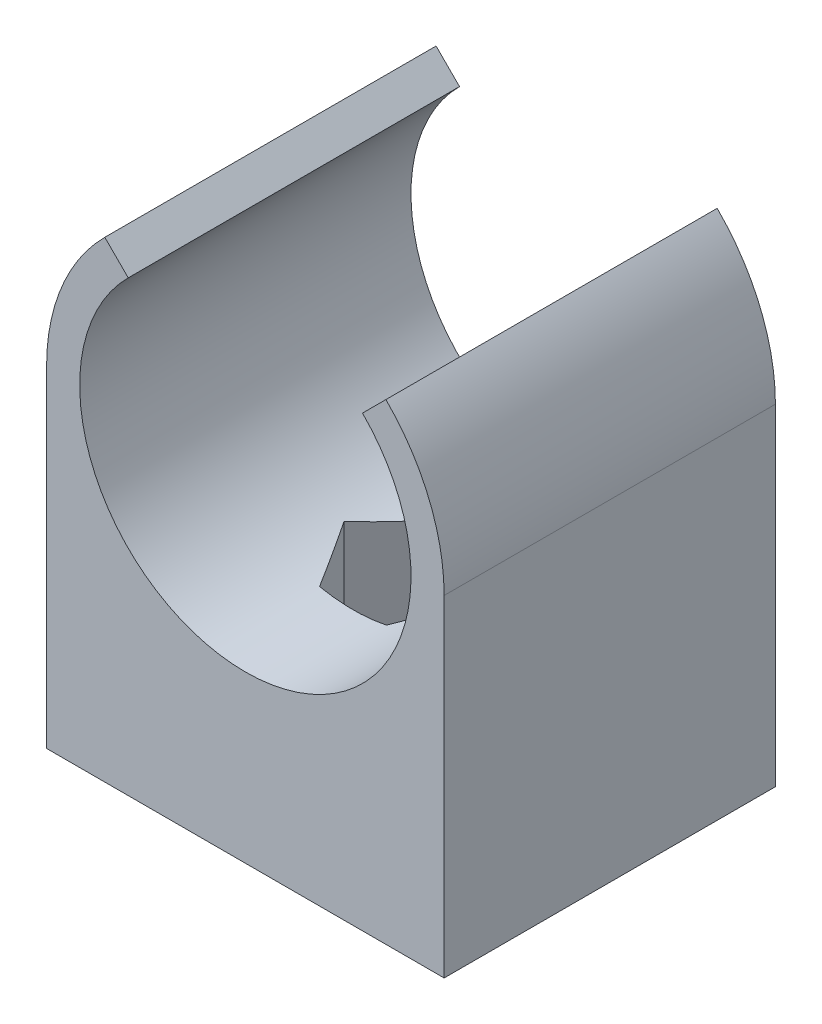
SolidWorks part; units mm, degrees
material "PP 共聚物"
ref_plane "前视基准面" through (0, 0, 0) normal (0, 0, 1) x (1, 0, 0)
ref_plane "上视基准面" through (0, 0, 0) normal (0, 1, 0) x (1, 0, 0)
ref_plane "右视基准面" through (0, 0, 0) normal (1, 0, 0) x (0, 0, -1)
sketch "草图1" plane through (0, 0, 0) normal (0, 0, 1) x (1, 0, 0)
  line L0 (-12, 10) -> (-12, 20)
  line L2 (-12, 10) -> (-12, 0)
  line L3 (-12, 0) -> (12, 0)
  line L4 (12, 10) -> (12, 0)
  line L5 (-7.0711, 27.0711) -> (-8.4853, 28.4853)
  line L6 (0, 41.9292) -> (0, 30) construction
  line L7 (12, 10) -> (12, 20)
  line L8 (7.0711, 27.0711) -> (8.4853, 28.4853)
  line L11 (0, 20) -> (0, -7.785) construction
  arc A0 (-7.0711, 27.0711) -> (7.0711, 27.0711) centre (0, 20) ccw
  arc A1 (-8.4853, 28.4853) -> (-12, 20) centre (0, 20) ccw
  arc A2 (12, 20) -> (8.4853, 28.4853) centre (0, 20) ccw
  dimension "D4" = 20
  dimension "D1" = 10
  dimension "D2" = 24
  dimension "D3" = 12
  dimension "D5" = 45
  dimension "D6" = 45
extrude "凸台-拉伸1" add sketch "草图1" along normal blind 20
hole_wizard "Ø5.0 (5) 直径孔1" positions "草图5" profile "草图6" hole size "Ø5.0" standard "Gb" end condition through all
sketch "草图5" plane through (0, 0, 0) normal (0, -1, 0) x (-1, 0, 0)
  line L0 (-12, -20) -> (-12, 0) construction
  line L2 (12, -20) -> (-12, -20) construction
  point P0 (0, -10)
  dimension "D1" = 12
  dimension "D2" = 10
sketch "草图6" plane through (0, 0, 10) normal (1, 0, 0) x (0, 0, -1)
  line L0 (0, 0) -> (0, 28.4853)
  line L1 (0, 28.4853) -> (2.5, 28.4853)
  line L2 (2.5, 28.4853) -> (2.5, 0)
  line L5 (2.5, 0) -> (0, 0)
  line L11 (0, -6.35) -> (0, 107.95) construction
  dimension "通孔孔直径" = 5
  dimension "通孔孔深度" = 28.4853
ref_plane "基准面1" through (0, 10, 0) normal (0, -1, 0) x (-1, 0, 0)
sketch "草图7" plane through (0, 10, 0) normal (0, -1, 0) x (-1, 0, 0)
  line L1 (4.0415, -10) -> (2.0207, -6.5)
  line L2 (2.0207, -6.5) -> (-2.0207, -6.5)
  line L3 (-2.0207, -6.5) -> (-4.0415, -10)
  line L4 (-4.0415, -10) -> (-2.0207, -13.5)
  line L5 (-2.0207, -13.5) -> (2.0207, -13.5)
  line L6 (2.0207, -13.5) -> (4.0415, -10)
  circle A0 centre (0, -10) radius 3.5 construction
  dimension "D1" = 7
extrude "切除-拉伸3" cut sketch "草图7" against normal blind 5 and the other way blind 5 contours L3 L4 L5 L6 L1 L2
